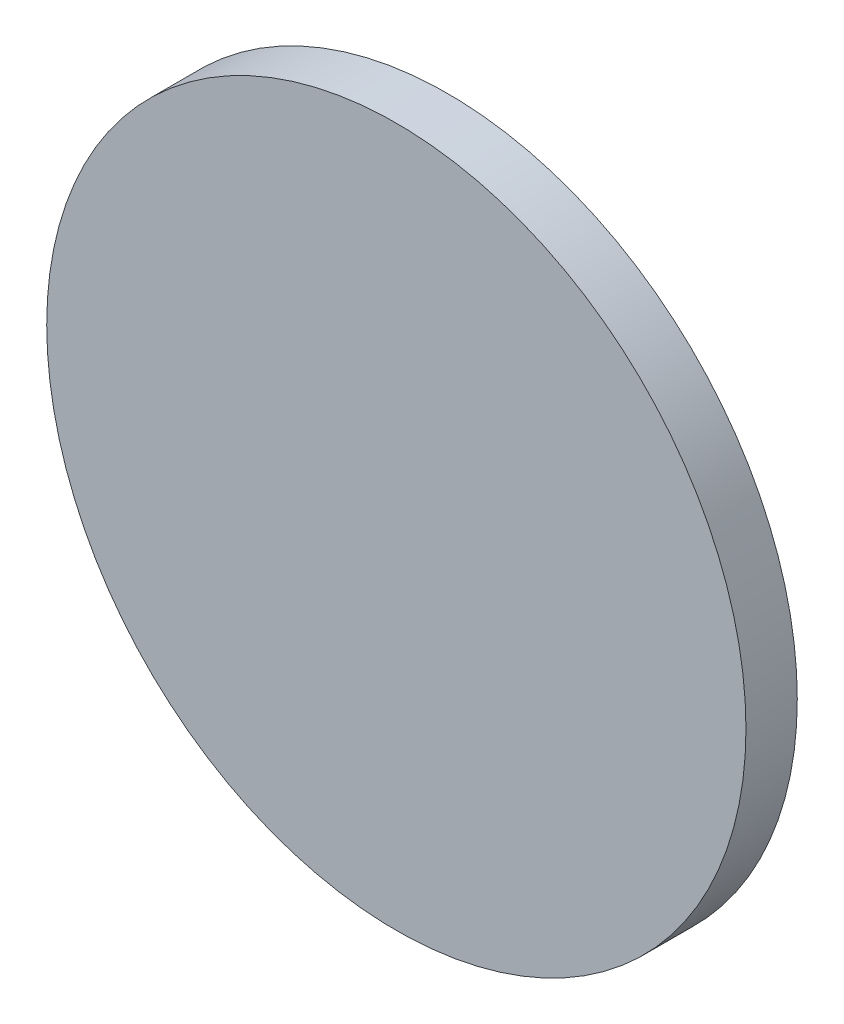
SolidWorks part; units mm, degrees
material "有机玻璃 (TM) GS 丙烯酸铸钣"
ref_plane "前视基准面" through (0, 0, 0) normal (0, 0, 1) x (1, 0, 0)
ref_plane "上视基准面" through (0, 0, 0) normal (0, 1, 0) x (1, 0, 0)
ref_plane "右视基准面" through (0, 0, 0) normal (1, 0, 0) x (0, 0, -1)
sketch "草图1" plane through (0, 0, 0) normal (0, 0, 1) x (1, 0, 0)
  circle A0 centre (0, 0) radius 27.25
  dimension "D1" = 54.5
extrude "凸台-拉伸1" add sketch "草图1" along normal blind 4
